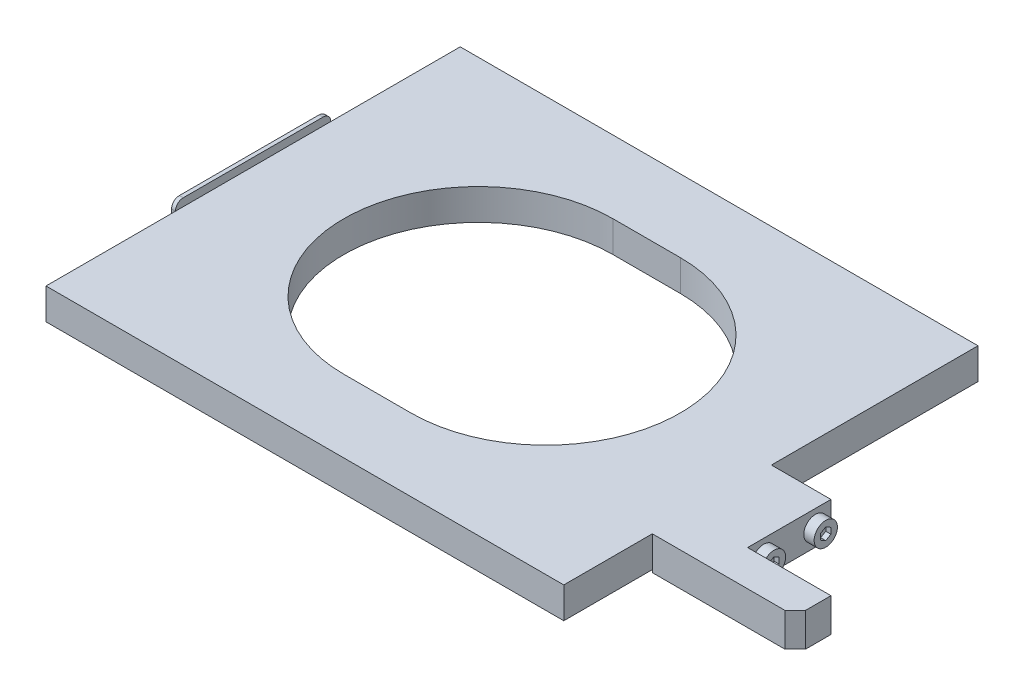
from build123d import *

# Parameters (mm, degrees)
EXTRUDE_1_DEPTH      = 50
EXTRUDE_1_DEPTH_BACK = 50
SKETCH_1_W           = 80
SKETCH_1_H           = 6
EXTRUDE_2_DEPTH      = 6.5
EXTRUDE_3_DEPTH      = 0.75
CUT_EXTRUDE_START    = 1
CUT_EXTRUDE_1_DEPTH  = 1
CUT_EXTRUDE_2_DEPTH  = 1
CUT_EXTRUDE_3_DEPTH  = 50
SKETCH_9_R           = 2.25
EXTRUDE_4_DEPTH      = 2
SKETCH_10_R          = 2.25
EXTRUDE_5_DEPTH      = 2
CUT_EXTRUDE_4_DEPTH  = 1
CUT_EXTRUDE_5_DEPTH  = 1


with BuildPart() as part:
    # 草图1 → 凸台-拉伸1 (new, two sides: drawn at the far end of the back side and taken through both)
    with BuildSketch(Plane(origin=(0, 0, 0), x_dir=(0, 0, -1), z_dir=(1, 0, 0)).offset(-EXTRUDE_1_DEPTH_BACK)):
        with Locations((0, 3)):
            Rectangle(SKETCH_1_W, SKETCH_1_H)
    extrude(amount=EXTRUDE_1_DEPTH + EXTRUDE_1_DEPTH_BACK)

    # 草图2 → 凸台-拉伸2 (add)
    with BuildSketch(Plane(origin=(0, 6, 0), x_dir=(-1, 0, 0), z_dir=(0, 1, 0))):
        Polygon((-50, -0.1), (-50, 22.9), (-75.6, 22.9), (-77.6, 20.9), (-77.6, 16), (-61.5, 16), (-61.5, -0.1), align=None)
    extrude(amount=-EXTRUDE_2_DEPTH)

    # 草图3 → 凸台-拉伸3 (add)
    with BuildSketch(Plane(origin=(-50, 0, 0), x_dir=(0, 0, -1), z_dir=(1, 0, 0))):
        with BuildLine():
            Line((-15, 6), (-15, -6))
            ThreePointArc((-15, -6), (-14.560660172, -7.060660172), (-13.5, -7.5))
            Line((-13.5, -7.5), (13.5, -7.5))
            ThreePointArc((13.5, -7.5), (14.560660172, -7.060660172), (15, -6))
            Line((15, -6), (15, 6))
            ThreePointArc((15, 6), (14.560660172, 7.060660172), (13.5, 7.5))
            Line((13.5, 7.5), (-13.5, 7.5))
            ThreePointArc((-13.5, 7.5), (-14.560660172, 7.060660172), (-15, 6))
        make_face()
        with BuildLine():
            Line((-12.5, -2.5), (12.5, -2.5))
            ThreePointArc((12.5, -2.5), (13.5, -1.5), (12.5, -0.5))
            Line((12.5, -0.5), (-12.5, -0.5))
            ThreePointArc((-12.5, -0.5), (-13.5, -1.5), (-12.5, -2.5))
        make_face(mode=Mode.SUBTRACT)
    extrude(amount=-EXTRUDE_3_DEPTH)

    # 草图4 → 旋转1 (revolve)
    with BuildSketch(Plane.XY.offset(-12), mode=Mode.PRIVATE) as revolve_1_sk:
        with BuildLine():
            Line((-51.75, 4), (-50.75, 4))
            Line((-50.75, 4), (-50.75, 2))
            Line((-50.75, 2), (-52.75, 2))
            ThreePointArc((-52.75, 2), (-52.381148113, 3.065574057), (-51.75, 4))
        make_face()
    revolve(revolve_1_sk.sketch.rotate(Axis((-50.75, 2, -12), (-1, 0, 0)), 270), axis=Axis((-50.75, 2, -12), (-1, 0, 0)))

    # 草图5 → 旋转2 (revolve)
    with BuildSketch(Plane.XY.offset(12), mode=Mode.PRIVATE) as revolve_2_sk:
        with BuildLine():
            Line((-51.75, 4), (-50.75, 4))
            Line((-50.75, 4), (-50.75, 2))
            Line((-50.75, 2), (-52.75, 2))
            ThreePointArc((-52.75, 2), (-52.381148113, 3.065574057), (-51.75, 4))
        make_face()
    revolve(revolve_2_sk.sketch.rotate(Axis((-50.75, 2, 12), (-1, 0, 0)), 270), axis=Axis((-50.75, 2, 12), (-1, 0, 0)))

    # 草图6 → 切除-拉伸1 (cut)
    with BuildSketch(Plane(origin=(-52.75, 0, 0), x_dir=(0, 0, -1), z_dir=(1, 0, 0)).offset(CUT_EXTRUDE_START)):
        with BuildLine():
            Line((-13.989974874, 1.8), (-12.2, 1.8))
            Line((-12.2, 1.8), (-12.2, 0.010025126))
            ThreePointArc((-12.2, 0.010025126), (-12, 0), (-11.8, 0.010025126))
            Line((-11.8, 0.010025126), (-11.8, 1.8))
            Line((-11.8, 1.8), (-10.010025126, 1.8))
            ThreePointArc((-10.010025126, 1.8), (-10, 2), (-10.010025126, 2.2))
            Line((-10.010025126, 2.2), (-11.8, 2.2))
            Line((-11.8, 2.2), (-11.8, 3.989974874))
            ThreePointArc((-11.8, 3.989974874), (-12, 4), (-12.2, 3.989974874))
            Line((-12.2, 3.989974874), (-12.2, 2.2))
            Line((-12.2, 2.2), (-13.989974874, 2.2))
            ThreePointArc((-13.989974874, 2.2), (-14, 2), (-13.989974874, 1.8))
        make_face()
    extrude(amount=-CUT_EXTRUDE_1_DEPTH, mode=Mode.SUBTRACT)

    # 草图7 → 切除-拉伸2 (cut)
    with BuildSketch(Plane(origin=(-52.75, 0, 0), x_dir=(0, 0, -1), z_dir=(1, 0, 0)).offset(CUT_EXTRUDE_START)):
        with BuildLine():
            Line((10.010025126, 1.8), (11.8, 1.8))
            Line((11.8, 1.8), (11.8, 0.010025126))
            ThreePointArc((11.8, 0.010025126), (12, 0), (12.2, 0.010025126))
            Line((12.2, 0.010025126), (12.2, 1.8))
            Line((12.2, 1.8), (13.989974874, 1.8))
            ThreePointArc((13.989974874, 1.8), (14, 2), (13.989974874, 2.2))
            Line((13.989974874, 2.2), (12.2, 2.2))
            Line((12.2, 2.2), (12.2, 3.989974874))
            ThreePointArc((12.2, 3.989974874), (12, 4), (11.8, 3.989974874))
            Line((11.8, 3.989974874), (11.8, 2.2))
            Line((11.8, 2.2), (10.010025126, 2.2))
            ThreePointArc((10.010025126, 2.2), (10, 2), (10.010025126, 1.8))
        make_face()
    extrude(amount=-CUT_EXTRUDE_2_DEPTH, mode=Mode.SUBTRACT)

    # 草图8 → 切除-拉伸3 (cut)
    with BuildSketch(Plane(origin=(0, 0, 0), x_dir=(-1, 0, 0), z_dir=(0, 1, 0))):
        with BuildLine():
            Line((6.5, 26), (-6.5, 26))
            ThreePointArc((-6.5, 26), (-32.5, 0), (-6.5, -26))
            Line((-6.5, -26), (6.5, -26))
            ThreePointArc((6.5, -26), (32.5, 0), (6.5, 26))
        make_face()
    extrude(amount=CUT_EXTRUDE_3_DEPTH, mode=Mode.SUBTRACT)

    # 草图9 → 凸台-拉伸4 (add)
    with BuildSketch(Plane(origin=(61.5, 0, 0), x_dir=(0, 0, -1), z_dir=(1, 0, 0))):
        with Locations((-2.9, 2.75)):
            Circle(SKETCH_9_R)
    extrude(amount=EXTRUDE_4_DEPTH)

    # 草图10 → 凸台-拉伸5 (add)
    with BuildSketch(Plane(origin=(61.5, 0, 0), x_dir=(0, 0, -1), z_dir=(1, 0, 0))):
        with Locations((-12.9, 2.75)):
            Circle(SKETCH_10_R)
    extrude(amount=EXTRUDE_5_DEPTH)

    # 草图11 → 切除-拉伸4 (cut)
    with BuildSketch(Plane(origin=(63.5, 0, 0), x_dir=(0, 0, -1), z_dir=(1, 0, 0))):
        Polygon((-1.9, 3.327350269), (-2.9, 3.904700538), (-3.9, 3.327350269), (-3.9, 2.172649731), (-2.9, 1.595299462), (-1.9, 2.172649731), align=None)
    extrude(amount=-CUT_EXTRUDE_4_DEPTH, mode=Mode.SUBTRACT)

    # 草图12 → 切除-拉伸5 (cut)
    with BuildSketch(Plane(origin=(63.5, 0, 0), x_dir=(0, 0, -1), z_dir=(1, 0, 0))):
        Polygon((-11.9, 3.327350269), (-12.9, 3.904700538), (-13.9, 3.327350269), (-13.9, 2.172649731), (-12.9, 1.595299462), (-11.9, 2.172649731), align=None)
    extrude(amount=-CUT_EXTRUDE_5_DEPTH, mode=Mode.SUBTRACT)


solid = part.part
